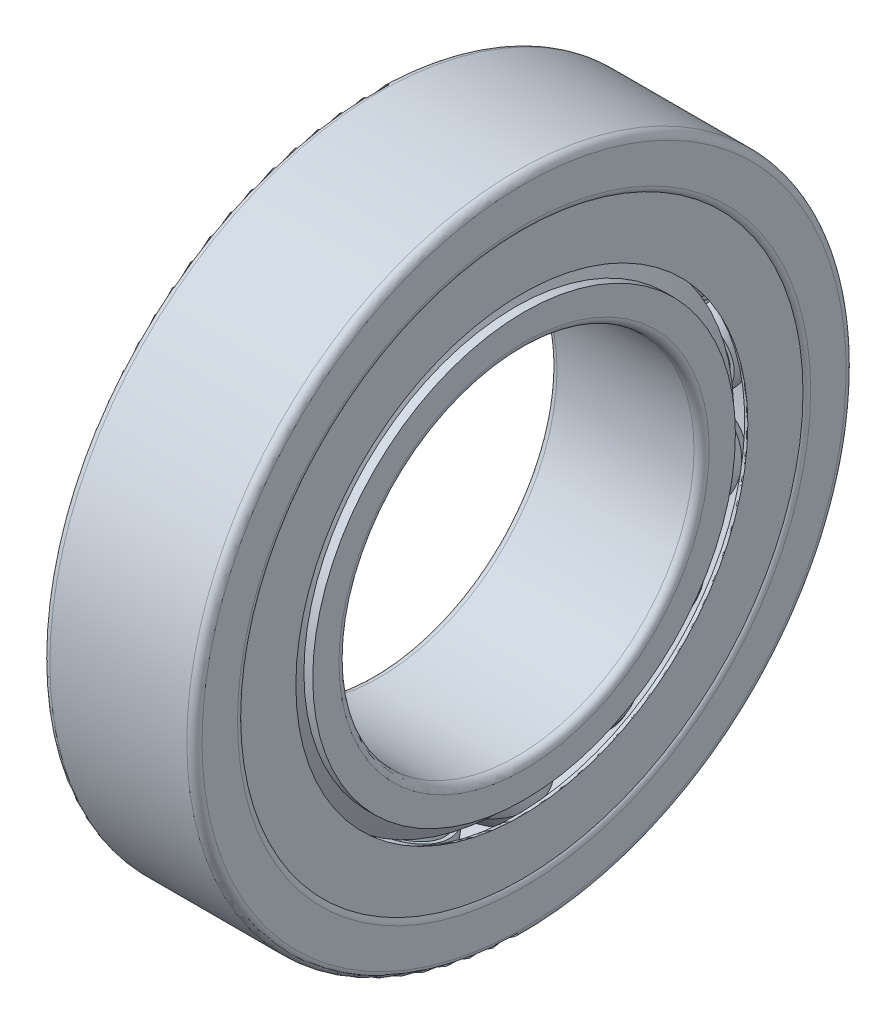
from build123d import *
from build123d.topology import SkipClean

# Parameters (mm, degrees)
SKETCH5_W         = 1.7999999999999998
SKETCH5_H         = 1.1999999999999993
CIRPATTERN5_COUNT = 17
CIRPATTERN2_COUNT = 17


with BuildPart() as part:
    # Sketch2 → Revolve1 (revolve)
    with BuildSketch(Plane.XY, mode=Mode.PRIVATE) as revolve1_sk:
        with BuildLine():
            Line((4.533333333333332, 18.000000000000004), (5.303133692252827, 16.66666666666667))
            Line((5.303133692252827, 16.66666666666667), (5.999999999999998, 16.66666666666667))
            Line((5.999999999999998, 16.66666666666667), (5.999999999999998, 14.600000000000003))
            ThreePointArc((5.999999999999998, 14.600000000000003), (5.824264068711927, 14.175735931288076), (5.399999999999999, 14.000000000000004))
            Line((5.399999999999999, 14.000000000000004), (-5.4, 14.000000000000002))
            ThreePointArc((-5.4, 14.000000000000002), (-5.824264068711929, 14.175735931288076), (-6, 14.600000000000003))
            Line((-6, 14.600000000000003), (-6, 16.66666666666667))
            Line((-6, 16.66666666666667), (-5.303133692252829, 16.66666666666667))
            Line((-5.303133692252829, 16.66666666666667), (-4.533333333333333, 18.000000000000004))
            Line((-4.533333333333333, 18.000000000000004), (-2.2360679774997916, 18.000000000000004))
            ThreePointArc((-2.2360679774997916, 18.000000000000004), (-8.4e-16, 17), (2.23606797749979, 18.000000000000004))
            Line((2.23606797749979, 18.000000000000004), (4.533333333333332, 18.000000000000004))
        make_face()
        with BuildLine():
            Line((-6, 25.4), (-6.000000000000002, 22.599999999999994))
            ThreePointArc((-6.000000000000002, 22.599999999999994), (-5.824264068711929, 22.17573593128807), (-5.400000000000002, 22))
            Line((-5.400000000000002, 22), (-2.236067977499787, 22.000000000000004))
            ThreePointArc((-2.236067977499787, 22.000000000000004), (-8.4e-16, 23), (2.2360679774997845, 22.000000000000004))
            Line((2.2360679774997845, 22.000000000000004), (5.400000000000016, 22.000000000000007))
            ThreePointArc((5.400000000000016, 22.000000000000007), (5.824264068711952, 22.17573593128808), (6.000000000000033, 22.600000000000012))
            Line((6.000000000000033, 22.600000000000012), (5.9999999999999964, 25.4))
            ThreePointArc((5.9999999999999964, 25.4), (5.824264068711925, 25.824264068711926), (5.399999999999999, 25.999999999999996))
            Line((5.399999999999999, 25.999999999999996), (-5.400000000000002, 25.999999999999996))
            ThreePointArc((-5.400000000000002, 25.999999999999996), (-5.824264068711929, 25.824264068711926), (-6, 25.4))
        make_face()
    revolve(revolve1_sk.sketch.rotate(Axis((-3.4999999999999996, 0, 0), (1, 0, 0)), 90), axis=Axis((-3.4999999999999996, 0, 0), (1, 0, 0)))


with BuildPart() as body_2:
    # Sketch5 → Revolve3 (revolve)
    with BuildSketch(Plane.XY, mode=Mode.PRIVATE) as revolve3_sk:
        with Locations((-1.7e-16, 20)):
            Rectangle(SKETCH5_W, SKETCH5_H)
    revolve(revolve3_sk.sketch.rotate(Axis((-19.927092192426834, 0, 0), (1, 0, 0)), 90), axis=Axis((-19.927092192426834, 0, 0), (1, 0, 0)))



with BuildPart() as body_3:
    # Sketch3 → Revolve2 (revolve)
    with BuildSketch(Plane.XY):
        with BuildLine():
            Line((-3.3000000000000007, 20), (3.3000000000000007, 20))
            ThreePointArc((3.3000000000000007, 20), (-8.3e-16, 23.3), (-3.3000000000000007, 20))
        make_face()
    revolve(axis=Axis((-3.3000000000000007, 20, 0), (1, 0, 0)))


with BuildPart() as cirpattern5_1:
    # CirPattern5: pattern copy
    add(body_3.part.rotate(Axis((0, -6.6e-16, 1.2e-16), (1, 0, 0)), 1 * 360 / CIRPATTERN5_COUNT))


with BuildPart() as cirpattern5_2:
    # CirPattern5: pattern copy
    add(body_3.part.rotate(Axis((0, -6.6e-16, 1.2e-16), (1, 0, 0)), 2 * 360 / CIRPATTERN5_COUNT))


with BuildPart() as cirpattern5_3:
    # CirPattern5: pattern copy
    add(body_3.part.rotate(Axis((0, -6.6e-16, 1.2e-16), (1, 0, 0)), 3 * 360 / CIRPATTERN5_COUNT))


with BuildPart() as cirpattern5_4:
    # CirPattern5: pattern copy
    add(body_3.part.rotate(Axis((0, -6.6e-16, 1.2e-16), (1, 0, 0)), 4 * 360 / CIRPATTERN5_COUNT))


with BuildPart() as cirpattern5_5:
    # CirPattern5: pattern copy
    add(body_3.part.rotate(Axis((0, -6.6e-16, 1.2e-16), (1, 0, 0)), 5 * 360 / CIRPATTERN5_COUNT))


with BuildPart() as cirpattern5_6:
    # CirPattern5: pattern copy
    add(body_3.part.rotate(Axis((0, -6.6e-16, 1.2e-16), (1, 0, 0)), 6 * 360 / CIRPATTERN5_COUNT))


with BuildPart() as cirpattern5_7:
    # CirPattern5: pattern copy
    add(body_3.part.rotate(Axis((0, -6.6e-16, 1.2e-16), (1, 0, 0)), 7 * 360 / CIRPATTERN5_COUNT))


with BuildPart() as cirpattern5_8:
    # CirPattern5: pattern copy
    add(body_3.part.rotate(Axis((0, -6.6e-16, 1.2e-16), (1, 0, 0)), 8 * 360 / CIRPATTERN5_COUNT))


with BuildPart() as cirpattern5_9:
    # CirPattern5: pattern copy
    add(body_3.part.rotate(Axis((0, -6.6e-16, 1.2e-16), (1, 0, 0)), 9 * 360 / CIRPATTERN5_COUNT))


with BuildPart() as cirpattern5_10:
    # CirPattern5: pattern copy
    add(body_3.part.rotate(Axis((0, -6.6e-16, 1.2e-16), (1, 0, 0)), 10 * 360 / CIRPATTERN5_COUNT))


with BuildPart() as cirpattern5_11:
    # CirPattern5: pattern copy
    add(body_3.part.rotate(Axis((0, -6.6e-16, 1.2e-16), (1, 0, 0)), 11 * 360 / CIRPATTERN5_COUNT))


with BuildPart() as cirpattern5_12:
    # CirPattern5: pattern copy
    add(body_3.part.rotate(Axis((0, -6.6e-16, 1.2e-16), (1, 0, 0)), 12 * 360 / CIRPATTERN5_COUNT))


with BuildPart() as cirpattern5_13:
    # CirPattern5: pattern copy
    add(body_3.part.rotate(Axis((0, -6.6e-16, 1.2e-16), (1, 0, 0)), 13 * 360 / CIRPATTERN5_COUNT))


with BuildPart() as cirpattern5_14:
    # CirPattern5: pattern copy
    add(body_3.part.rotate(Axis((0, -6.6e-16, 1.2e-16), (1, 0, 0)), 14 * 360 / CIRPATTERN5_COUNT))


with BuildPart() as cirpattern5_15:
    # CirPattern5: pattern copy
    add(body_3.part.rotate(Axis((0, -6.6e-16, 1.2e-16), (1, 0, 0)), 15 * 360 / CIRPATTERN5_COUNT))


with BuildPart() as cirpattern5_16:
    # CirPattern5: pattern copy
    add(body_3.part.rotate(Axis((0, -6.6e-16, 1.2e-16), (1, 0, 0)), 16 * 360 / CIRPATTERN5_COUNT))


with BuildPart() as cut_revolve1_tool:
    # Sketch6 → Cut-Revolve1 (revolve)
    with BuildSketch(Plane.XY):
        with BuildLine():
            Line((-3.2449961479175924, 20.599999999999998), (3.2449961479175924, 20.599999999999998))
            ThreePointArc((3.2449961479175924, 20.599999999999998), (-8.3e-16, 23.300000000000004), (-3.2449961479175924, 20.599999999999998))
        make_face()
        with BuildLine():
            Line((-3.2449961479175924, 19.400000000000006), (3.2449961479175924, 19.400000000000006))
            ThreePointArc((3.2449961479175924, 19.400000000000006), (-8.3e-16, 16.7), (-3.2449961479175924, 19.400000000000006))
        make_face()
    revolve(axis=Axis((-19.927092192426834, 0, 0), (1, 0, 0)))


with BuildPart() as part_1:
    add(part.part)

    # Cut-Revolve1: cut by cut_revolve1_tool
    add(cut_revolve1_tool.part, mode=Mode.SUBTRACT)

    # Sketch9 → Revolve5 (revolve)
    with BuildSketch(Plane.XY, mode=Mode.PRIVATE) as revolve5_sk:
        with BuildLine():
            Line((5.400000000000016, 22.000000000000007), (5.400000000000009, 17.999999999999996))
            ThreePointArc((5.400000000000009, 17.999999999999996), (5.629610059419066, 17.954327719506786), (5.824264068711945, 17.824264068711944))
            Line((5.824264068711945, 17.824264068711944), (5.824264068711952, 22.175735931288077))
            ThreePointArc((5.824264068711952, 22.175735931288077), (5.629610059419073, 22.045672280493235), (5.400000000000016, 22.000000000000007))
        make_face()
        with BuildLine():
            Line((-5.824264068711954, 22.175735931288077), (-5.824264068711947, 17.824264068711944))
            ThreePointArc((-5.824264068711947, 17.824264068711944), (-5.629610059419068, 17.954327719506786), (-5.400000000000011, 17.999999999999996))
            Line((-5.400000000000011, 17.999999999999996), (-5.400000000000017, 22.000000000000007))
            ThreePointArc((-5.400000000000017, 22.000000000000007), (-5.6296100594190746, 22.045672280493235), (-5.824264068711954, 22.175735931288077))
        make_face()
    revolve(revolve5_sk.sketch.rotate(Axis((-19.927092192426834, 0, 0), (1, 0, 0)), 90), axis=Axis((-19.927092192426834, 0, 0), (1, 0, 0)))


with BuildPart() as body_3_1:
    add(body_3.part)

    # Cut-Revolve1: cut by cut_revolve1_tool
    add(cut_revolve1_tool.part, mode=Mode.SUBTRACT)


with BuildPart() as cirpattern5_1_1:
    add(cirpattern5_1.part)

    # Cut-Revolve1: cut by cut_revolve1_tool
    add(cut_revolve1_tool.part, mode=Mode.SUBTRACT)


with BuildPart() as cirpattern5_2_1:
    add(cirpattern5_2.part)

    # Cut-Revolve1: cut by cut_revolve1_tool
    add(cut_revolve1_tool.part, mode=Mode.SUBTRACT)


with BuildPart() as cirpattern5_3_1:
    add(cirpattern5_3.part)

    # Cut-Revolve1: cut by cut_revolve1_tool
    add(cut_revolve1_tool.part, mode=Mode.SUBTRACT)


with BuildPart() as cirpattern5_4_1:
    add(cirpattern5_4.part)

    # Cut-Revolve1: cut by cut_revolve1_tool
    add(cut_revolve1_tool.part, mode=Mode.SUBTRACT)


with BuildPart() as cirpattern5_5_1:
    add(cirpattern5_5.part)

    # Cut-Revolve1: cut by cut_revolve1_tool
    add(cut_revolve1_tool.part, mode=Mode.SUBTRACT)


with BuildPart() as cirpattern5_6_1:
    add(cirpattern5_6.part)

    # Cut-Revolve1: cut by cut_revolve1_tool
    add(cut_revolve1_tool.part, mode=Mode.SUBTRACT)


with BuildPart() as cirpattern5_7_1:
    add(cirpattern5_7.part)

    # Cut-Revolve1: cut by cut_revolve1_tool
    add(cut_revolve1_tool.part, mode=Mode.SUBTRACT)


with BuildPart() as cirpattern5_8_1:
    add(cirpattern5_8.part)

    # Cut-Revolve1: cut by cut_revolve1_tool
    add(cut_revolve1_tool.part, mode=Mode.SUBTRACT)


with BuildPart() as cirpattern5_9_1:
    add(cirpattern5_9.part)

    # Cut-Revolve1: cut by cut_revolve1_tool
    add(cut_revolve1_tool.part, mode=Mode.SUBTRACT)


with BuildPart() as cirpattern5_10_1:
    add(cirpattern5_10.part)

    # Cut-Revolve1: cut by cut_revolve1_tool
    add(cut_revolve1_tool.part, mode=Mode.SUBTRACT)


with BuildPart() as cirpattern5_11_1:
    add(cirpattern5_11.part)

    # Cut-Revolve1: cut by cut_revolve1_tool
    add(cut_revolve1_tool.part, mode=Mode.SUBTRACT)


with BuildPart() as cirpattern5_12_1:
    add(cirpattern5_12.part)

    # Cut-Revolve1: cut by cut_revolve1_tool
    add(cut_revolve1_tool.part, mode=Mode.SUBTRACT)


with BuildPart() as cirpattern5_13_1:
    add(cirpattern5_13.part)

    # Cut-Revolve1: cut by cut_revolve1_tool
    add(cut_revolve1_tool.part, mode=Mode.SUBTRACT)


with BuildPart() as cirpattern5_14_1:
    add(cirpattern5_14.part)

    # Cut-Revolve1: cut by cut_revolve1_tool
    add(cut_revolve1_tool.part, mode=Mode.SUBTRACT)


with BuildPart() as cirpattern5_15_1:
    add(cirpattern5_15.part)

    # Cut-Revolve1: cut by cut_revolve1_tool
    add(cut_revolve1_tool.part, mode=Mode.SUBTRACT)


with BuildPart() as cirpattern5_16_1:
    add(cirpattern5_16.part)

    # Cut-Revolve1: cut by cut_revolve1_tool
    add(cut_revolve1_tool.part, mode=Mode.SUBTRACT)


with BuildPart() as body_2_1:
    with SkipClean():  # the faces are left unmerged after this step: merging them gives an invalid solid
        add(body_2.part)

        add(body_3_1.part)  # Revolve4 merges body 3
        # Sketch7 → Revolve4 (revolve)
        with BuildSketch(Plane.XY):
            with BuildLine():
                Line((-3, 20), (3, 20))
                ThreePointArc((3, 20), (-8.4e-16, 23), (-3, 20))
            make_face()
        revolve4 = revolve(axis=Axis((-3, 20, 0), (1, 0, 0)))

    # CirPattern2: Revolve4 ×17 about axis
    cirpattern2_axis = Axis((0, -6.6e-16, -1.2e-16), (1, 0, 0))
    for i in range(1, CIRPATTERN2_COUNT):
        add(revolve4.rotate(cirpattern2_axis, i * 360 / CIRPATTERN2_COUNT))


solid = Compound([part_1.part, cirpattern5_1_1.part, cirpattern5_2_1.part, cirpattern5_3_1.part, cirpattern5_4_1.part, cirpattern5_5_1.part, cirpattern5_6_1.part, cirpattern5_7_1.part, cirpattern5_8_1.part, cirpattern5_9_1.part, cirpattern5_10_1.part, cirpattern5_11_1.part, cirpattern5_12_1.part, cirpattern5_13_1.part, cirpattern5_14_1.part, cirpattern5_15_1.part, cirpattern5_16_1.part, body_2_1.part])
